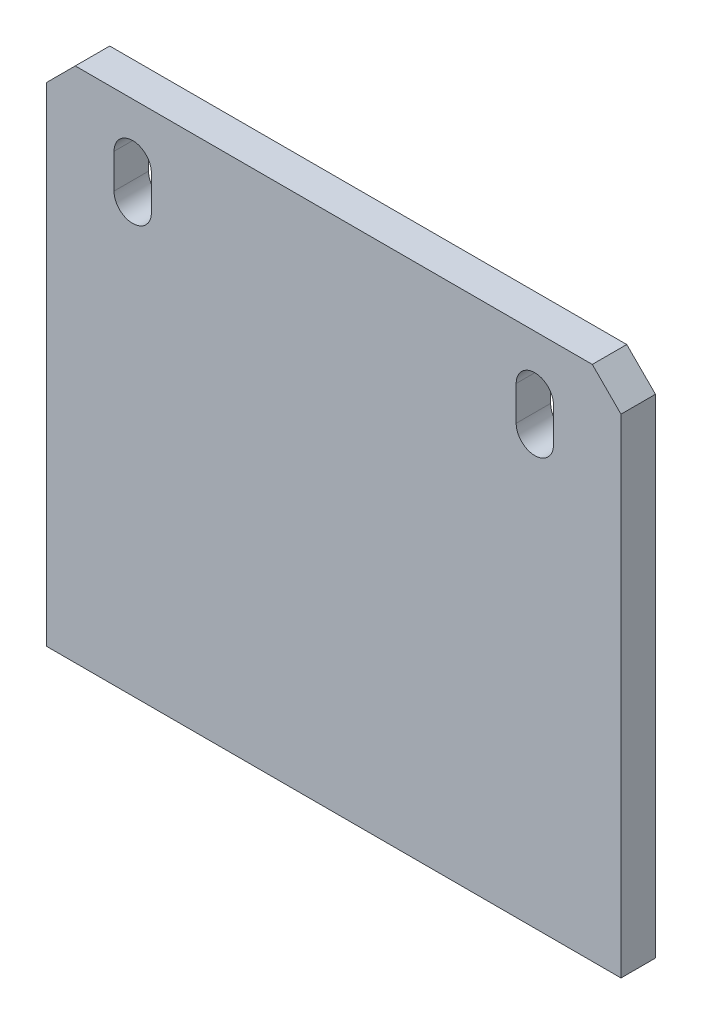
from build123d import *

# Parameters (mm, degrees)
SKETCH1_W           = 200
SKETCH1_H           = 180
BOSS_EXTRUDE1_DEPTH = 12
CHAMFER1_SIZE       = 10
CUT_EXTRUDE1_DEPTH  = 12


with BuildPart() as part:
    # Sketch1 → Boss-Extrude1 (new body)
    with BuildSketch(Plane.XY):
        Rectangle(SKETCH1_W, SKETCH1_H)
    extrude(amount=BOSS_EXTRUDE1_DEPTH)

    # Chamfer1
    chamfer1_edges = [part.edges().sort_by_distance(p)[0] for p in [
        (100, 90, 6),
        (-100, 90, 6),
    ]]
    chamfer(chamfer1_edges, length=CHAMFER1_SIZE)

    # Sketch2 → Cut-Extrude1 (cut)
    with BuildSketch(Plane.XY.offset(12)):
        with BuildLine():
            Line((-63.5, 71), (-63.5, 59))
            ThreePointArc((-63.5, 59), (-70, 52.5), (-76.5, 59))
            Line((-76.5, 59), (-76.5, 71))
            ThreePointArc((-76.5, 71), (-70, 77.5), (-63.5, 71))
        make_face()
        with BuildLine():
            Line((76.5, 71), (76.5, 59))
            ThreePointArc((76.5, 59), (70, 52.5), (63.5, 59))
            Line((63.5, 59), (63.5, 71))
            ThreePointArc((63.5, 71), (70, 77.5), (76.5, 71))
        make_face()
    extrude(amount=-CUT_EXTRUDE1_DEPTH, mode=Mode.SUBTRACT)


solid = part.part
